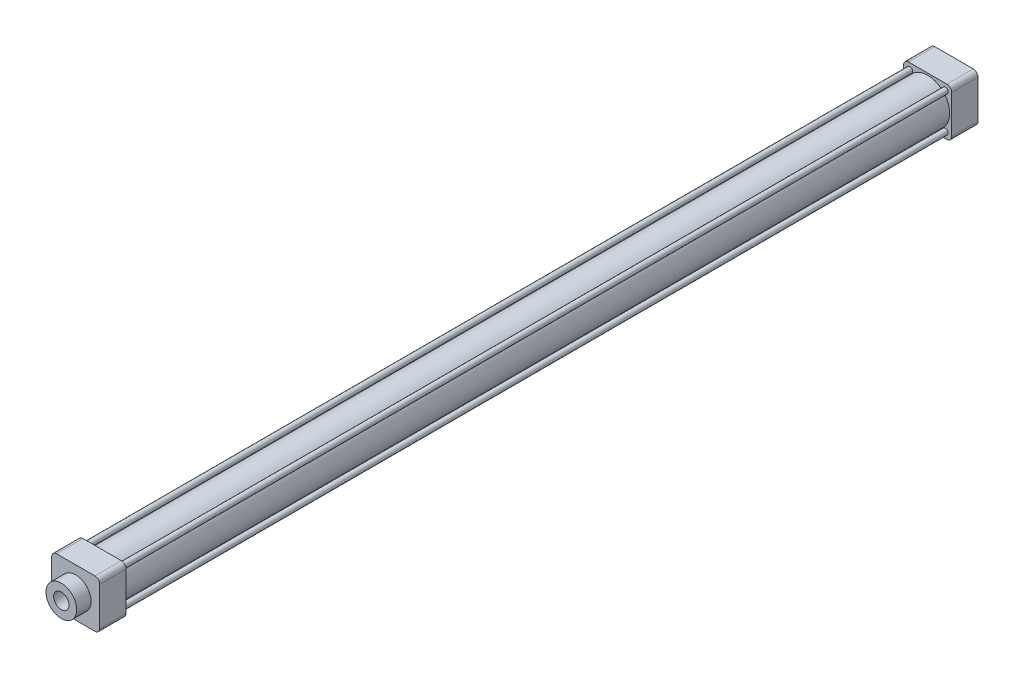
from build123d import *

# Parameters (mm, degrees)
SKETCH1_W           = 50
SKETCH1_H           = 50
BOSS_EXTRUDE1_DEPTH = 27.5
SKETCH2_R           = 23
SKETCH2_R_2         = 20
BOSS_EXTRUDE2_DEPTH = 860
SKETCH3_W           = 50
SKETCH3_H           = 50
BOSS_EXTRUDE3_DEPTH = 27.5
SKETCH4_R           = 16
BOSS_EXTRUDE4_DEPTH = 15
SKETCH5_R           = 8
CUT_EXTRUDE1_DEPTH  = 100
SKETCH6_R           = 3
BOSS_EXTRUDE5_DEPTH = 915
FILLET1_R           = 5


with BuildPart() as part:
    # Sketch1 → Boss-Extrude1 (new body)
    with BuildSketch(Plane.XY):
        Rectangle(SKETCH1_W, SKETCH1_H)
    extrude(amount=BOSS_EXTRUDE1_DEPTH)

    # Sketch2 → Boss-Extrude2 (add)
    with BuildSketch(Plane.XY.offset(27.5)):
        Circle(SKETCH2_R)
        Circle(SKETCH2_R_2, mode=Mode.SUBTRACT)
    extrude(amount=BOSS_EXTRUDE2_DEPTH)

    # Sketch3 → Boss-Extrude3 (add)
    with BuildSketch(Plane.XY.offset(887.5)):
        Rectangle(SKETCH3_W, SKETCH3_H)
    extrude(amount=BOSS_EXTRUDE3_DEPTH)

    # Sketch4 → Boss-Extrude4 (add)
    with BuildSketch(Plane.XY.offset(915)):
        Circle(SKETCH4_R)
    extrude(amount=BOSS_EXTRUDE4_DEPTH)

    # Sketch5 → Cut-Extrude1 (cut)
    with BuildSketch(Plane.XY.offset(930)):
        Circle(SKETCH5_R)
    extrude(amount=-CUT_EXTRUDE1_DEPTH, mode=Mode.SUBTRACT)

    # Sketch6 → Boss-Extrude5 (add)
    with BuildSketch(Plane.XY.offset(915)):
        with Locations((-18.5, 18.5)):
            Circle(SKETCH6_R)
        with Locations((18.5, 18.5)):
            Circle(SKETCH6_R)
        with Locations((18.5, -18.5)):
            Circle(SKETCH6_R)
        with Locations((-18.5, -18.5)):
            Circle(SKETCH6_R)
    extrude(amount=-BOSS_EXTRUDE5_DEPTH)

    # Fillet1
    fillet1_edges = [part.edges().sort_by_distance(p)[0] for p in [
        (25, -25, 901.25),
        (25, 25, 901.25),
        (-25, 25, 901.25),
        (-25, -25, 901.25),
        (25, -25, 13.75),
        (-25, -25, 13.75),
        (-25, 25, 13.75),
        (25, 25, 13.75),
    ]]
    fillet(fillet1_edges, radius=FILLET1_R)


solid = part.part
